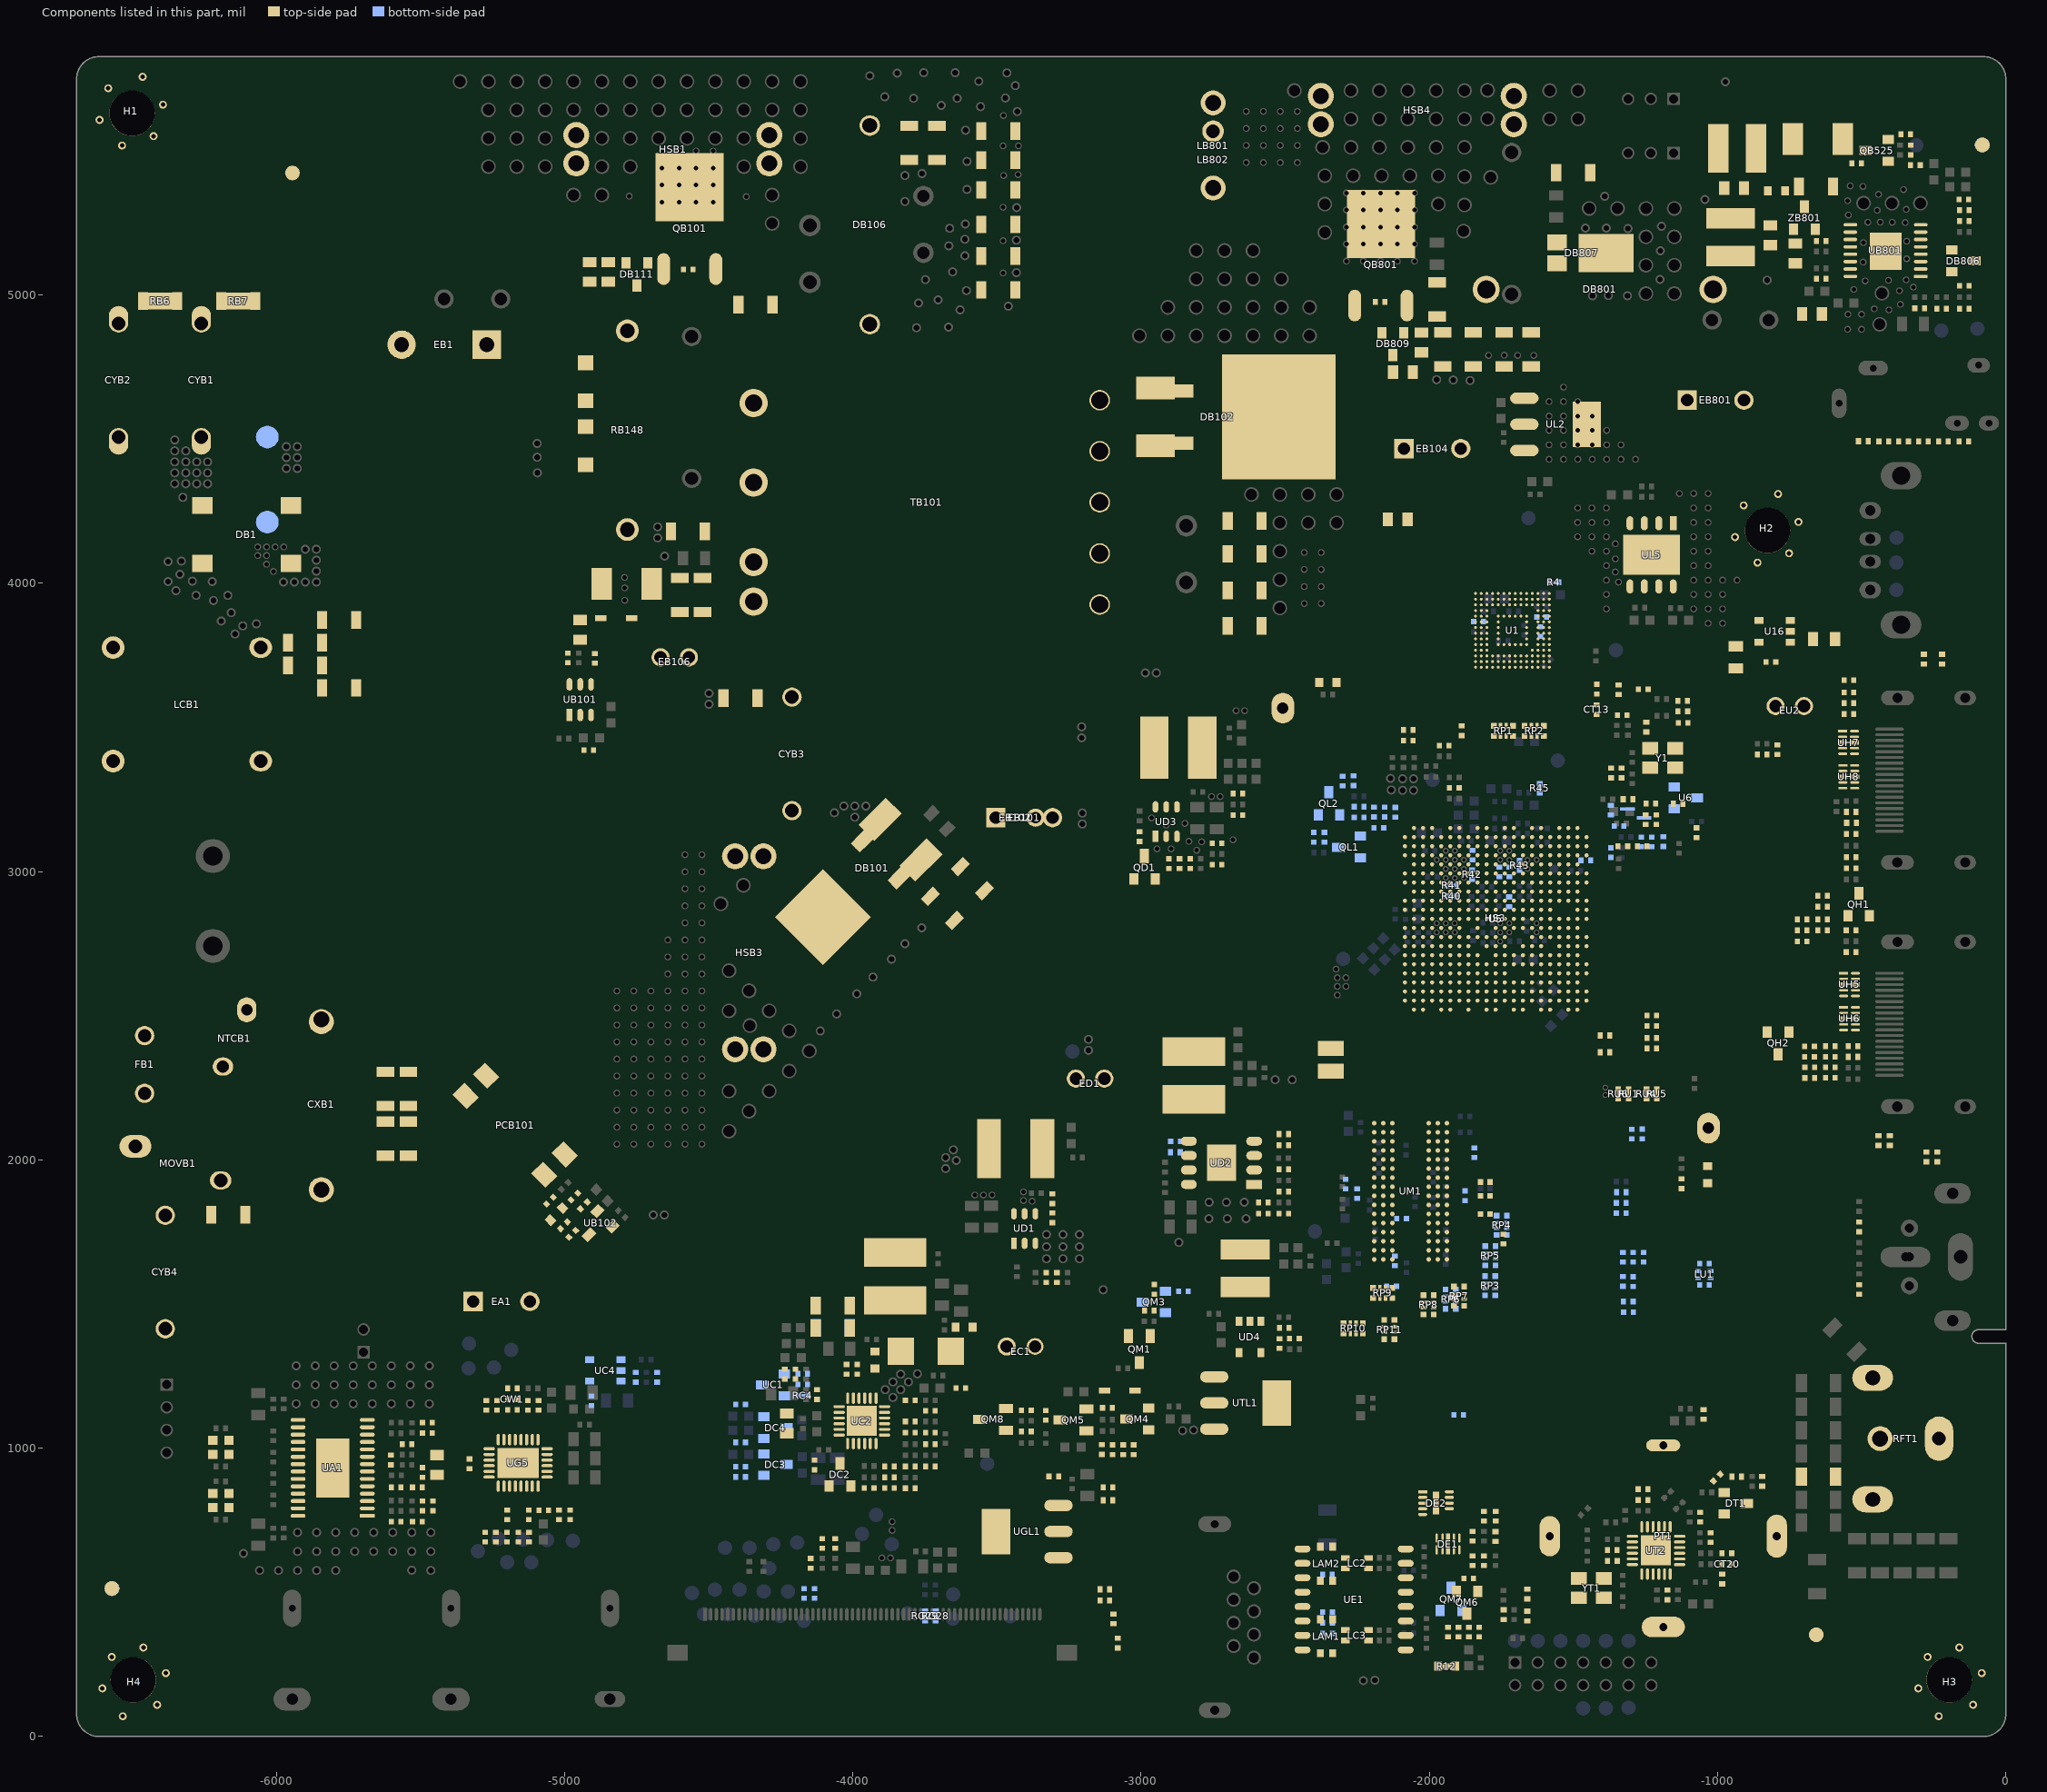
[diagram p0: the components of this part, seen from the top]
# Altium PCB MISC84395.PcbDoc (part 7 of 26)
Units mil, origin at the board's own origin, x right, y up, seen from the top; angles counter-clockwise.
Board outline 6692.91 x 5826.77 mil, 2 copper layers (TopLayer, BottomLayer), stack 61.855 mil thick; 951 components, 565 nets, 4374 pads, 1804 vias.
Unrouted connection lines stored in the file: 1.

## Part data (continued)
"Conformal Coating": library part 三防漆,25kg/Can,Peters
CT13: library part 0.022uF-0402-X7R-±10%-16V-D
CT20: library part 5.6pF-0402-NPO-±5%-50V-D
CT60: library part 4700pF-1206-X7R-±10%-1000V-D
CU CU1: library part 10uF-0805-X5R-+15%-16V-D
CW1: library part 004.003.0000503-D, "Ceramic capacitor,CAP MC,50V,1000pF,±10%,X7R,0402,SMD,TP-D"
CXB1: library part "X电容,CAP X2,MP,275VAC,0.47uF,±10%,S,15mm-Mini,PC,DIP,BM-DHMI", "CAP"
CYB1 CYB2 CYB3 CYB4: library part "Y电容,CAP Y1,CD,470pF,400VAC,±20%,KS,10mm,Y5U,DIP,Walsin-DHMI", "Y1 capacitor"
D4 D5 DK1: library part SFI0402-240E-2R5PP-LF-D
D11 D12 D13 D14 DH1 DH2 DH3 DH4 DH5 DH6 DI1 DI2 DI4 DI04 DK3 DO1 DO7 DT2 DT3 DV1 DV2 DV3 DV4: library part AVLC18S02003-D
DA1 DA2 DT4 DU1 DU2 DU3 DU4 DU5 DU6 DU7 DU8 DU9: library part AIES12U020R2-D
DB1: library part 004.005.0000860-D, "Bridge rectifier,DIO BRD,3A,800V,YBS,SMD,YBS3010A,YJ-D"
DB101: library part MBRB10150CT(GOOD-ARK)-D, "Diode"
DB102: library part "整流二极管,DIO FRD D1,10A,400V,TO-263,SMD,MURB1040CT,GOOD-ARK-D", "Diode"
DB104 DB802: library part M7(WEJ)-D, "Diode"
DB106: library part FR107(编带/LRC)-DLAI, "Diode"
DB109 DB110: library part "整流二极管,DIO FRD S,1.2A,800V,eSGA,SMD,R12K,GOOD-ARK-D"
DB111 DB806 DB809: library part LBAV70LT1G(LRC)-D, "Diode"
DB121: library part BAV21WS-D, "Diode"
DB801: library part SR310(编带/台半)-DLMI, "Diode"
DB807: library part TSPB5H150S-D, "Diode"
DC1: library part SK34A-SMA-F-D
DC2 DC3 DC4: library part BAT54S-D
DE1: library part RCLAMP0524P-TCT-D, "RCLAMP0524J"
DE2: library part "TVS管,DIO ESD,3.6pF,18V,DFN2525P10E,SMD,AZ3133-04F,Amazing（OEM物料）-D"
DM1: library part 1N4148WS-D
DT1: library part BAV99-BR-D
EA1: library part 470uF-16V±20%-10×12-105℃-编带-F=5.0-XL-DHAI
EB1: library part 100uF-450V-±20%-18×41-105℃-KS-折脚开槽(CapXon)-S对策-DLMI, "Electrolytic"
EB101: library part 470uF-25V-±20%-10×12.5-105℃-GF-编带-F=5.0(CapXon)-DHAI, "Electrolytic"
EB102: library part 270uF-16V-±20%-8×11.5-105℃-PS-短脚-F=3.5(Capxon), "Solid-state"
EB104: library part 330uF-35V-±20%-10×12.5-105℃-GF-编带-F=5.0(Capxon)-DHAI, "Electrolytic"
EB106: library part 10uF-50V-±20%-5×11-105℃-GH-编带-F=2.5(CapXon)-DHAI, "Electrolytic"
EB801: library part 100uF-63V-±20%-10×12.5-105℃-GF-编带-F=5.0(CapXon)-DHAI, "Electrolytic"
EC1: library part 100uF-35V-±20%-6.3×11-105℃-KF-编带-F=2.5(CapXon)-DHAI, "Electrolytic"
ED1: library part 470uF-10V-±20%-6.3×11-105℃-黑底白字-编带-F=2.5-XF-DHAI, "Electrolytic"
EU2: library part 100uF-16V-±20%-5×11-105℃-黑底白字-编带-F=2.5-XF-DHAI, "Electrolytic"
EVA1 EVA2 EVA3 EVA4 EVA5 EVA6: library part 7×7×3mm-C-4305防火泡棉-黑色-DLMI, "EVA"
FB1: library part 004.026.0000010-DHMI, "Slow-blow fuse,FUSE T,P,3.15A,250VAC,8.5×4.0×8mm,DIP,TP,Walter-DHMI"
GD1 GD2 GD3 GD4: library part 7.00×8.35mm-尼龙-白色-WQM-DHMI, "Mylar stud"
GL1 GL2: library part 005.002.0000011, "Silicone,0.2g,general,60,white,SLD-8854W,XY-DHMI"
GND_JP1 GND_JP2: library part GND
H1 H2 H3 H4: library part "Location hole-D"
HS3: library part 004.040.0002110-DLMI, "Heat sink,AL6063,40.0×40.0×2.3mm,black,nano-carbon,wave-pattern type-bottom milled groove,Asink-DLMI"
HSB1 HSB3 HSB4: library part 004.040.0006600-DHMI, "Heat sink,17.5×14.5×0.5mm,copper sheet,matte tin plated,natural,four pins,WT-DHMI"
L3: library part GZ1005U121CTF(120ohm-500mA)-D
LAM1 LAM2: library part PKG-003494/P000077171, "Common-mode choke,60uH,2.0mm,SMD,sunlord-D"
LB801: library part SYDR1212-L003-EDL-DHMI, "I-core inductor"
LB802: library part 差模电感,Inductor,DR12×14,68uH,0.45,20Ts,H13.5MAX,SYDR1214-L068uA,DIP,Soldier-DHMI, "I-core inductor"
LB804 LB805: library part 004.004.0001664, "Power inductor,2.2uH,±20%,2A,0.28×1P,DR4.5×3.2,SMD,CD43-2.2uH,wenshan-D"
LBA1 LBA2 LBA3 LBA4: library part 004.004.0000327-D, "Ferrite bead,BEAD,120ohm,0603,600mA,SMD,TP,FCM1608KF-121T06-D"
LC1: library part SCD54TL-6R8M-D
LC2 LC3: library part 004.004.0002112, "Common-mode choke,2012,800Ω,1.2mm,WCM2012F2SF-801-N,SMD,TAI-TECH-D"
LCB1: library part SYUU10.5-L002-JM-DHMI, "Common mode"
LD1: library part SWPA6045S4R7MT-D
LD2 LD3: library part SCD54TL-2R2M-D
LD5: library part 004.004.0001664-D, "Power inductor,2.2uH,±20%,2A,0.28×1P,DR4.5×3.2,SMD,CD43-2.2uH,wenshan-D"
LG02 LT20: library part FCM1005KF-121T06(120ohm-500mA)-D
LT1: library part MGHB1005S102T-LF-D
LT2: library part SDCL1005CR33JTDF-D
LT5 LT6: library part "SDCL1005C33NJTDF(顺络) -D"
LU1: library part DLP11SN900HL2-D, "CHOKE COIL COMMON MODE 100MA Z0=90ohm"
M1 M2 M3 M4 M5 M6: library part MARK-D
MAC: library part Barcode
ML1: library part MALAY
MOVB1: library part TVR10561KSW(为勤)-DHMI, "Varistor"
MR300 MR301: library part 56ohm-0402-±5%-1/16W-D
MR313 R50: library part 240ohm-0402-±1%-1/16W-D
NTCB1: library part SCK102R55AMBY502(短脚/为勤)-DHMI, "Thermistor"
P1: library part "导电硅胶,3×2×2.5mm,Black,Silicone Rubber,SMD,Joinset", "EVA"
PCB101: library part LTV-817S-TA-B(光宝)-DMI, "Optocoupler"
PT1: library part 004.040.0000768-DMI, "Shield can,tinplate,natural,20.3×16.3×6mm,with sealing,LHD-DMI"
QB101: library part 场效应管,NMOS,5.2,650V,1.02ohm@ID=2.6A@VGS=10V,DPAK,TK5P65W,TOSHIBA-D, "N Channel Single MOSFET"
QB525: library part LMBT3904LT1G-D-NPN, "Q-NPN-#-#-#"
QB801: library part ME15N10(松木)-D, "N Channel Single MOSFET"
QD1: library part 2N7002K-7(DIODES)-D
QH1 QH2: library part MMBT3904(f≥350MHz)-D-NPN, "Q-NPN-#-#-#"
QL1 QL2 QM3 QM4 QM6 QM7: library part KMBT3904-D
QM1 QM5 QM8: library part ME2325-G-D, "MOS-P"
R1 R2 RT2 RT4: library part 004.002.0000568-D, "Thick film resistor,RES,1/16W,100ohm,±5%,0402,SMD-D"
R3 R5 R38 R39 R53 R54 R55 R56 RC5 RC8 RC19 RC20 RC23 RF1 RG6 RI1 RI7 RI11 RT14: library part 0ohm-0402-±5%-1/16W-D
R4 R40 R41 R42 R43 R45 RC4 RG28 RG29 RU1 RU4 RU5 RU6: library part 0ohm-0402-PCB-D, "0ohm-0402-PCB-D"
R9 R10 RC24 RD6 RG24 RG30 RK3 RK5 RK6 RK7 RK8 RM7 RM9 RT7 RT9: library part 10Kohm-0402-±5%-1/16W-D
R11 RG1 RG2 RG3 RG4 RG5 RG79 RG80 RG81 RG82 RG84 RG85 RG87 RG89 RG91 RH6 RH7 RH9 RH16 RH17: library part 22ohm-0402-±5%-1/16W-D
R12: library part 0ohm-0603-PCB-D, "0ohm-0603-PCB-D"
R21 R28 RA5 RA6 RA12 RA13 RB801 RH1 RH10 RK2 RL7 RL9: library part 1Kohm-0402-±5%-1/16W-D
R26 RO45: library part 180ohm-0402-±5%-1/16W-D
R27: library part 11Kohm-0402-±1%-1/16W-D
R30 R33 R34 R37 RA31 RD3 RD24 RD40 RK12 RL2 RL3 RL4 RL5 RL6 RL8 RL12 RM2 RM3 RM4 RM8 RT34 RT36 RT39 RT40 RU3 RU7 RU9 RU10 RU12 RV15 RV17: library part 4K7ohm-0402-±5%-1/16W-D
R46 R47 R48 R49 R51 R52 RB132: library part 1Kohm-0402-±1%-1/16W-D
RA8 RC6 RC10 RD2 RD25 RD26 RM5: library part 100Kohm-0402-±5%-1/16W-D
RA11: library part 12Kohm-0402-±5%-1/16W-D
RA19 RC13 RC18 RC27 RI9 RI12: library part 47Kohm-0402-±5%-1/16W-D
RA21: library part 20Kohm-0402-±1%-1/16W-D
RA25 RC36: library part 10ohm-0402-±5%-1/16W-D
RA27 RB809 RC1: library part 10ohm-0805-±5%-1/8W-D
RA32 RL10 RL11 RM1: library part 4k7ohm-0402-±5%-1/16W-D
RB1 RB2 RB3 RB4: library part 1M2ohm-1206-±5%-1/4W-D, "RES"
RB5 RB101 RB102: library part 330Kohm-1206-±5%-1/4W-D, "RES"
RB6 RB7: library part 0ohm-1206-PCB-D, "0ohm-1206-PCB-D"
RB103 RB109 RB133: library part 10Kohm-0402-±1%-1/16W-D
RB104: library part 47Kohm-0402-±1%-1/16W-D
RB105: library part 510ohm-0402-±1%-1/16W-D
RB106 RB121: library part 68ohm-0805-±5%-1/8W-D
RB107 RB807 RB824 RB825: library part 20ohm-0805-±5%-1/8W-D, "RES"
RB114: library part 4R7ohm-1206-±1%-1/4W-D, "RES"
RB115: library part 4R7ohm-1206-±5%-1/4W-D, "RES"
RB116 RB117 RB118 RB119 RB810 RB811 RB826 RB830 RB832 RB833 RB834 RB837: library part 10ohm-1206-±5%-1/4W-D, "RES"
RB124 RB125 RB126 RB136: library part 68ohm-1206-±5%-1/4W-D
RB128 RB129: library part 47ohm-1206-±5%-1/4W-D, "RES"
RB130: library part 20ohm-1206-±5%-1/4W-D
RB131: library part 1Kohm-0603-±1%-1/10W-D
RB134: library part 4K7ohm-0402-±1%-1/16W-D, "RES"
RB135: library part 18Kohm-0402-±1%-1/16W-D, "RES"
RB140: library part 51Kohm-0805-±1%-1/8W-D, "RES"
RB141 RB142: library part 2Mohm-1206-±5%-1/4W-D, "RES"
RB148: library part MOF-0R27ohm-±5%-2WS(编带/Futaba)-DLAI, "RES"
RB151 RB152 RB153 RB154 RB155 RB156: library part 100Kohm-1206-±5%-1/4W-D, "RES"
RB158: library part 3Kohm-0402-±1%-1/16W-D
RB802 RB808: library part 10Kohm-0402-±5%-1/16W-D, "RES"
RB803: library part 8K06ohm-0402-±1%-1/16W-D
RB804: library part 270ohm-0402-±5%-1/16W-D
RB805: library part 1Kohm-0402-±5%-1/16W-D, "R"
RB806: library part 30Kohm-0603-±5%-1/10W-D
RB812 RC7 RC9 RD1 RD7 RD12: library part 18Kohm-0402-±1%-1/16W-D
RB814: library part 004.002.0001276, "Thick film resistor,RES,1/8W,330Kohm,±1%,0805-Auto,SMD-D"
RB816: library part 2R2ohm-0805-±5%-1/8W-D
RB818 RB819 RB820 RB821: library part 0R68ohm-1206-±5%-1/4W-D
RB822 RD51: library part 15Kohm-0402-±1%-1/16W-D
RB827: library part 560kohm-0402-±1%-1/16W-D
RC2: library part 12Kohm-0402-±1%-1/16W-D
RC3: library part 1K2ohm-0402-±1%-1/16W-D
RC11 RC28: library part 10ohm-0603-±5%-1/10W-D
RC12: library part 56Kohm-0402-±1%-1/16W-D
RC14: library part 4R7ohm-0402-±5%-1/16W-D
RC15: library part 121Kohm-0402-±1%-1/16W-D
RC16: library part 470Kohm-0402-±1%-1/16W-D
RC17: library part 39Kohm-0402-±1%-1/16W-D, "RES"
RC21 RD50: library part 62Kohm-0402-±1%-1/16W-D
RC22: library part 7K5ohm-0402-±1%-1/16W-D
RC25: library part 100Kohm-0402-±1%-1/16W-D
RC26 RC29: library part 6K2ohm-0402-±1%-1/16W-D
RC31: library part 16Kohm-0402-±1%-1/16W-D
RC35: library part 9K1ohm-0402-±1%-1/16W-D
RD4: library part 3K3ohm-0402-±1%-1/16W-D
RD8: library part 30Kohm-0402-±1%-1/16W-D
RD9 RD27 RD28 RF2: library part 1Mohm-0402-±5%-1/16W-D
RD13: library part 300Kohm-0402-±1%-1/16W-D
RD15 RD16: library part 5K6ohm-0402-±1%-1/16W-D
RD17: library part 13Kohm-0402-±1%-1/16W-D
RD18 RD19 RH2 RH3 RH4 RH5 RH11 RH12 RH14 RH15 RI4 RK4 RK14 RT6 RV16 RV18: library part 100ohm-0402-±5%-1/16W-D
RE1 RE2 RE3 RE4: library part 75ohm-0402-±1%-1/16W-D
RE11 RE12 RE13 RE14: library part 2R2ohm-0402-±1%-1/16W-D
RFT1: library part "RF头,RF JACK,H,IEC,T14.5,CH6.3,12.4×13.2×7.7mm,DIP,LHD-020组件,LHD-DLMI", "T-IEC-6.3mm-#-#"
RG01 RG02 RL1 RM13 RM14: library part 004.002.0000558-D, "Thick film resistor,RES,1/16W,0ohm,±5%,0402,SMD-D"
RG7 RG9: library part 1Kohm-1206-±5%-1/4W-D
RG8: library part 470ohm-1206-±5%-1/4W-D, "RES"
RG17 RG18 RG19 RH8 RH18: library part 33ohm-0402-±5%-1/16W-D
RH13: library part 200ohm-0402-±5%-1/16W-D
RI5: library part 75ohm-0402-±5%-1/16W-D
RK1: library part 4K7ohm-0402-±1%-1/16W-D
RM10 RM11: library part 2Kohm-0402-±1%-1/16W-D
RM12 RM15: library part 004.002.0000578-D, "Thick film resistor,RES,1/16W,100Kohm,±1%,0402,SMD-D"
RO4: library part 120ohm-0402-±5%-1/16W-D
RP1 RP2: library part 4*22ohm-0402-±5%-1/16W-D
RP3 RP4 RP5 RP6 RP7 RP8 RP9 RP10 RP11: library part 4*0ohm-0402-±5%-1/16W-D
RS1 RS2: library part 0ohm-0603-±5%-1/10W-D
RT1: library part 750Kohm-0402-±5%-1/16W-D
RT5 RT10: library part 300ohm-0402-±25%-D
RU2 RU8: library part 5R1ohm-0402-±5%-1/16W-D
RW1 RW3: library part 004.002.0000488-D, "Thick film resistor,RES,1/16W,56Kohm,±1%,0402,SMD-D"
RW2: library part 004.002.0000104-D, "Thick film resistor,RES,1/16W,33Kohm,±1%,0402,SMD-D"
TB101: library part SYEQ2612-T002-JM-DLMI, "Transformer"
TP-TDT: library part TEST, "TEST"
U1: library part THGBMBG6D1KBAIL-D
U5: library part 004.016.0000830, "TV main chip,IC Main Chip,MSD6A348AT-X1,CAN TV,32bit,Multi-Core,BGA406,SMD,Mstar-D"
U6: library part SGM810-SXN3L-D
U16: library part "限流开关,IC OCP,1.0A,5.5V,SOT-23-5,SMD,APL3551CBI-TRG,ANPEC-D"
UA1: library part 004.012.0000275-D, "Audio amplifier,IC Audio AMP,Class D,2X8W@12V@8ohm,E-TSSOP-28L,SMD,AD52050B-26QG28NRR,ESMT-D"
UB101: library part 004.010.0000426, "PWM controller,IC PWM Controller,65KHZ,SOT23-6,SMD,OB2273C,ON-Bright-D"
UB102: library part AZ431AN-ATRE1(BCD)-D, "SMD 431"
UB801: library part MP3398AGF-Z(MPS)-D, "IC"
UC1: library part TL431G-AE2-R(UTC)-D
UC2: library part G5517-D
UC4: library part "运算放大器,IC OP Amplifier,1 channel,18MHz,TSOT23-5,SMD,ANX7003AAK,ANAX"
UD1 UD3: library part 004.010.0001029-D, "DC-DC chip,IC DC-DC,Syn,3A,18V,500kHz,SOT23-6,SMD,SY8113IADC,Silergy-D"
UD2: library part "DC-DCоƬ,IC DC-DC,Syn,5A,16V,600KHz,ESOP-8,SMD,MSH6110A,Mstar-D"
UD4: library part "DC-DCоƬ,IC DCDC,Syn,1.2A,7.0V,1.5MHz,SOT23-5,SMD,LC2127CB5TR,Leadchip-D"
UE1: library part H16101MC-D
UG5: library part 004.022.0000213-D, "LCD level-shift chip,IC Driver,TQFN4X5-28,SMD,G2595EKL1U-K,GMT-D"
UGL1 UL2 UTL1: library part LC1117CLTR33-D
UH5 UH6 UH7 UH8: library part ULC0524P-D, "RCLAMP0524J"
UL5: library part LC1118CS8TR1833-D
UM1: library part NT5CB256M16CP-DI-D
UT2: library part MxL661-D
Y1 YT1: library part 32MHz-±10PPM-12PF-SMD3225-JWT-D
ZB801: library part BZX84C24(蓝箭)-D, "Diode"
用于U5上: library part Φ12mm×12mm-黑色-125度(UL认证)-D